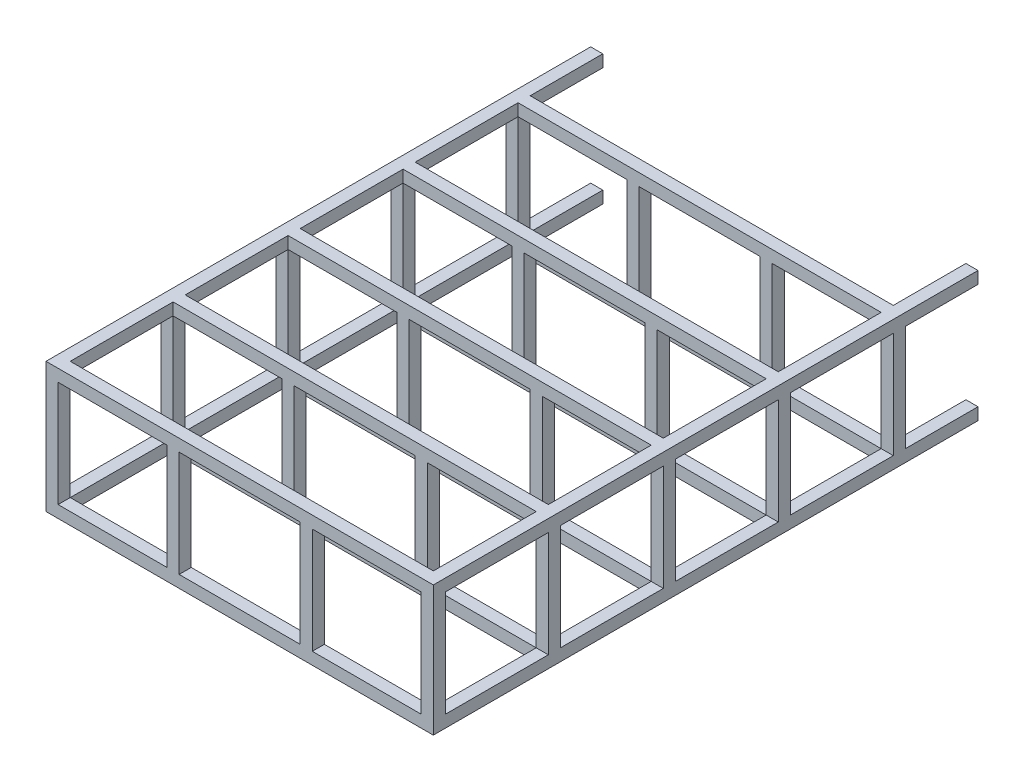
from build123d import *

# Parameters (mm, degrees)
SKETCH1_W                = 1280
SKETCH1_H                = 430
SKETCH1_W_2              = 360
SKETCH1_H_2              = 350
SKETCH1_W_3              = 400
BOSS_EXTRUDE1_DEPTH      = 40
BOSS_EXTRUDE2_DEPTH      = 1520
BOSS_EXTRUDE2_DEPTH_BACK = 280
SKETCH2_W                = 40
SKETCH2_H                = 40
SKETCH3_W                = 40
SKETCH3_H                = 40
BOSS_EXTRUDE3_DEPTH      = 411
SKETCH4_W                = 40
SKETCH4_H                = 40
BOSS_EXTRUDE4_DEPTH      = 1240
SKETCH5_W                = 40
SKETCH5_H                = 40
BOSS_EXTRUDE5_DEPTH      = 390


with BuildPart() as part:
    # Sketch1 → Boss-Extrude1 (new body)
    with BuildSketch(Plane.XY):
        with Locations((640, 215)):
            Rectangle(SKETCH1_W, SKETCH1_H)
        with Locations((220, 215)):
            Rectangle(SKETCH1_W_2, SKETCH1_H_2, mode=Mode.SUBTRACT)
        with Locations((1060, 215)):
            Rectangle(SKETCH1_W_2, SKETCH1_H_2, mode=Mode.SUBTRACT)
        with Locations((640, 215)):
            Rectangle(SKETCH1_W_3, SKETCH1_H_2, mode=Mode.SUBTRACT)
    extrude(amount=BOSS_EXTRUDE1_DEPTH)

    # Sketch2 → Boss-Extrude2 (add, two sides: drawn at the far end of the back side and taken through both)
    with BuildSketch(Plane.XY.offset(40).offset(-BOSS_EXTRUDE2_DEPTH_BACK)):
        with Locations((20, 410)):
            Rectangle(SKETCH2_W, SKETCH2_H)
        with Locations((20, 20)):
            Rectangle(SKETCH2_W, SKETCH2_H)
        with Locations((1260, 20)):
            Rectangle(SKETCH2_W, SKETCH2_H)
        with Locations((1260, 410)):
            Rectangle(SKETCH2_W, SKETCH2_H)
    extrude(amount=BOSS_EXTRUDE2_DEPTH + BOSS_EXTRUDE2_DEPTH_BACK)

    # Sketch3 → Boss-Extrude3 (add)
    with BuildSketch(Plane.XZ):
        with Locations((20, 400)):
            Rectangle(SKETCH3_W, SKETCH3_H)
        with Locations((1260, 400)):
            Rectangle(SKETCH3_W, SKETCH3_H)
        with Locations((20, 780)):
            Rectangle(SKETCH3_W, SKETCH3_H)
        with Locations((1260, 780)):
            Rectangle(SKETCH3_W, SKETCH3_H)
        with Locations((20, 1160)):
            Rectangle(SKETCH3_W, SKETCH3_H)
        with Locations((1260, 1160)):
            Rectangle(SKETCH3_W, SKETCH3_H)
        with Locations((20, 1540)):
            Rectangle(SKETCH3_W, SKETCH3_H)
        with Locations((1260, 1540)):
            Rectangle(SKETCH3_W, SKETCH3_H)
    extrude(amount=-BOSS_EXTRUDE3_DEPTH)

    # Sketch4 → Boss-Extrude4 (add)
    with BuildSketch(Plane.ZY):
        with Locations((20, 410)):
            Rectangle(SKETCH4_W, SKETCH4_H)
        with Locations((20, 20)):
            Rectangle(SKETCH4_W, SKETCH4_H)
        with Locations((400, 20)):
            Rectangle(SKETCH4_W, SKETCH4_H)
        with Locations((400, 410)):
            Rectangle(SKETCH4_W, SKETCH4_H)
        with Locations((780, 410)):
            Rectangle(SKETCH4_W, SKETCH4_H)
        with Locations((780, 20)):
            Rectangle(SKETCH4_W, SKETCH4_H)
        with Locations((1160, 20)):
            Rectangle(SKETCH4_W, SKETCH4_H)
        with Locations((1160, 410)):
            Rectangle(SKETCH4_W, SKETCH4_H)
        with Locations((1540, 410)):
            Rectangle(SKETCH4_W, SKETCH4_H)
        with Locations((1540, 20)):
            Rectangle(SKETCH4_W, SKETCH4_H)
    extrude(amount=-BOSS_EXTRUDE4_DEPTH)

    # Sketch5 → Boss-Extrude5 (add)
    with BuildSketch(Plane.XZ):
        with Locations((420, 20)):
            Rectangle(SKETCH5_W, SKETCH5_H)
        with Locations((860, 20)):
            Rectangle(SKETCH5_W, SKETCH5_H)
        with Locations((420, 400)):
            Rectangle(SKETCH5_W, SKETCH5_H)
        with Locations((860, 400)):
            Rectangle(SKETCH5_W, SKETCH5_H)
        with Locations((420, 780)):
            Rectangle(SKETCH5_W, SKETCH5_H)
        with Locations((860, 780)):
            Rectangle(SKETCH5_W, SKETCH5_H)
        with Locations((420, 1160)):
            Rectangle(SKETCH5_W, SKETCH5_H)
        with Locations((860, 1160)):
            Rectangle(SKETCH5_W, SKETCH5_H)
        with Locations((860, 1540)):
            Rectangle(SKETCH5_W, SKETCH5_H)
        with Locations((420, 1540)):
            Rectangle(SKETCH5_W, SKETCH5_H)
    extrude(amount=-BOSS_EXTRUDE5_DEPTH)


solid = part.part
